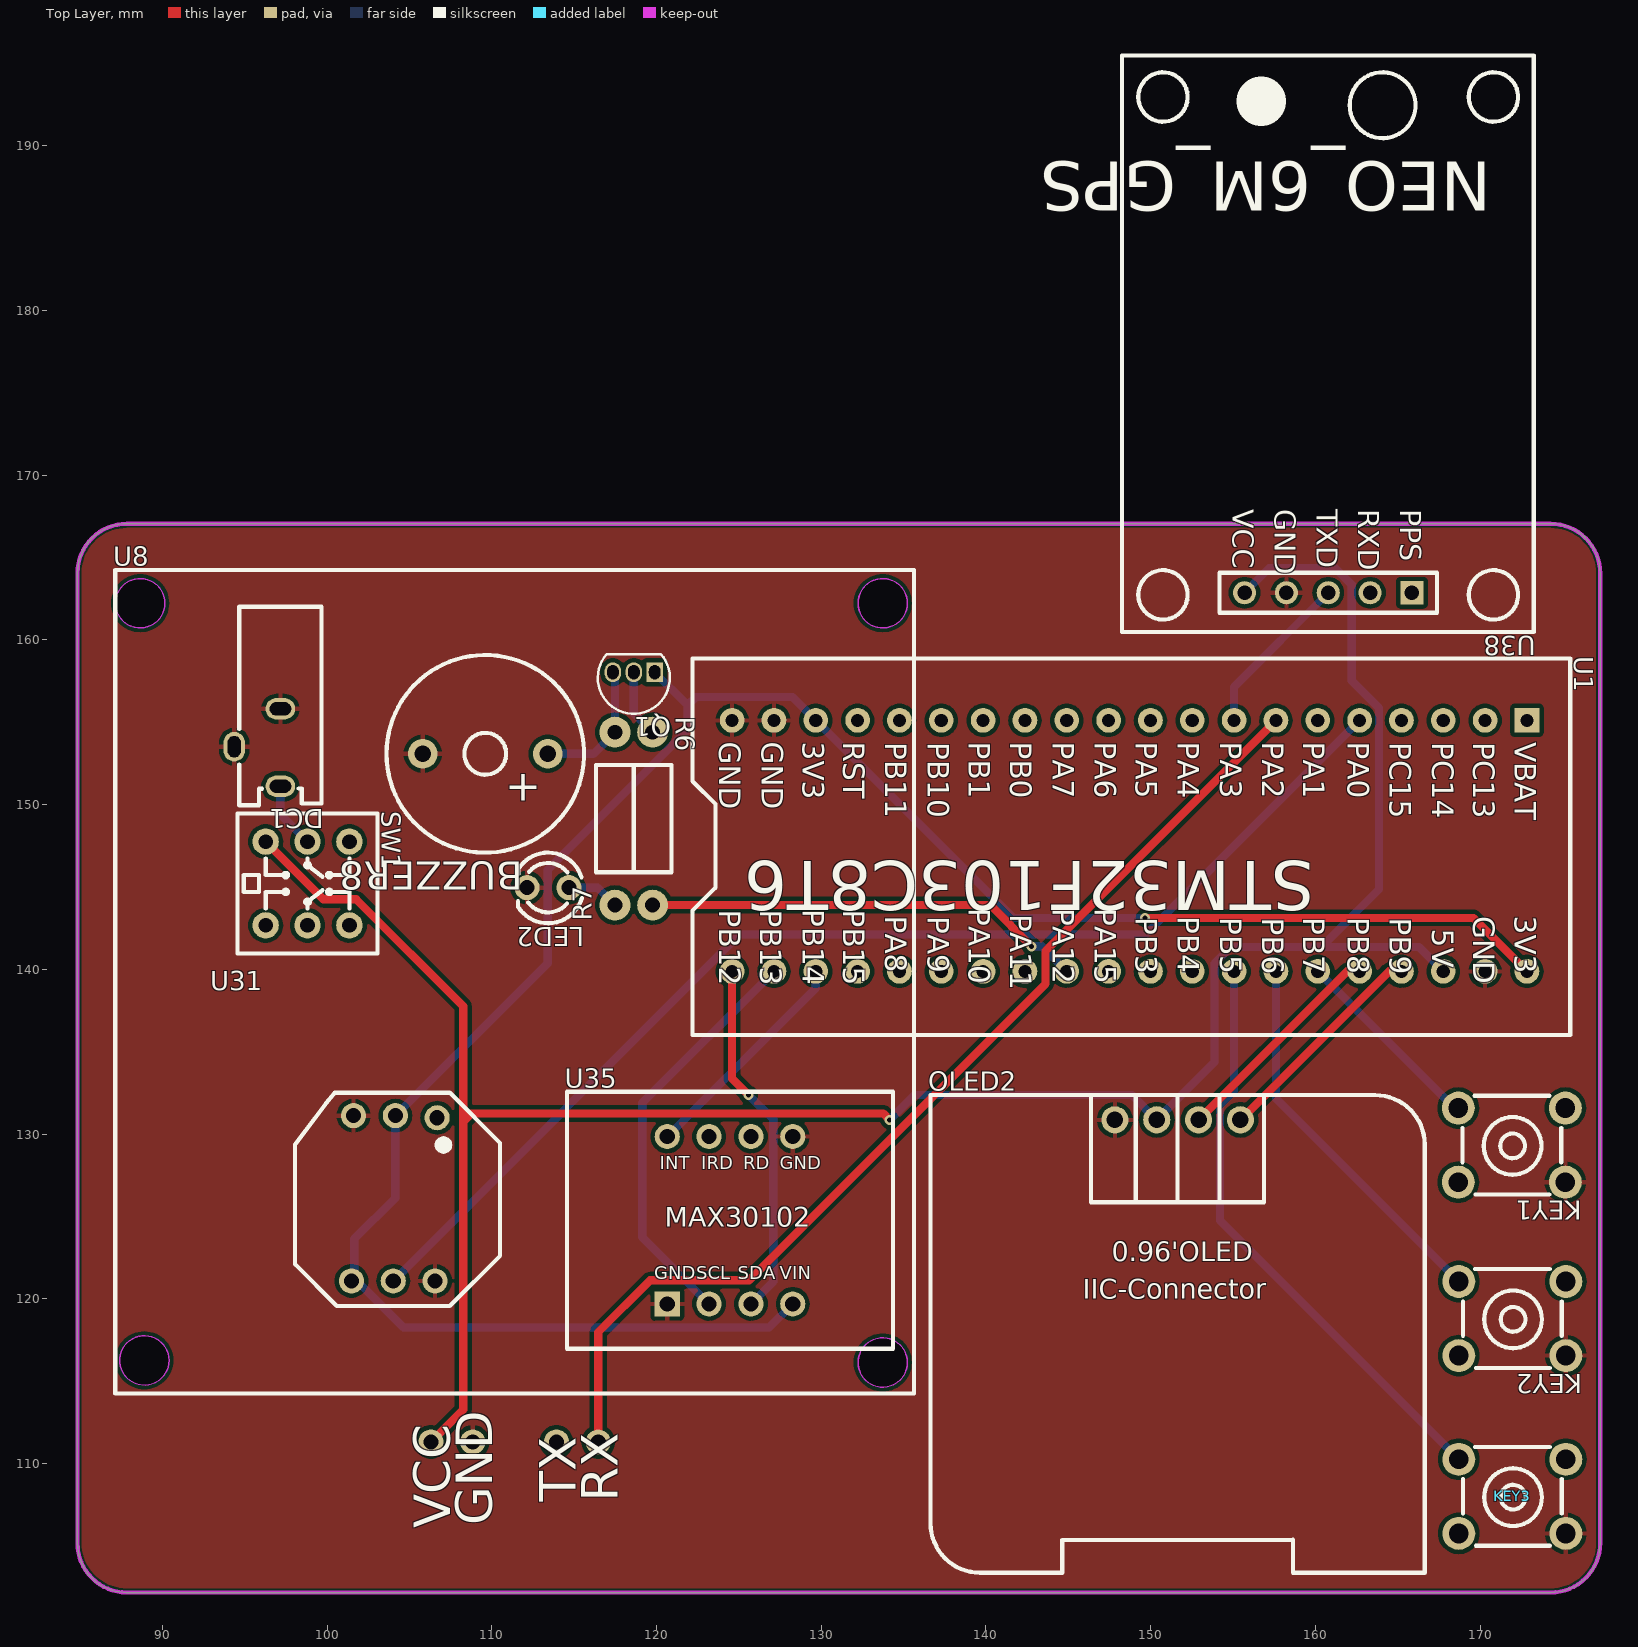
[diagram p0: Top Layer view]
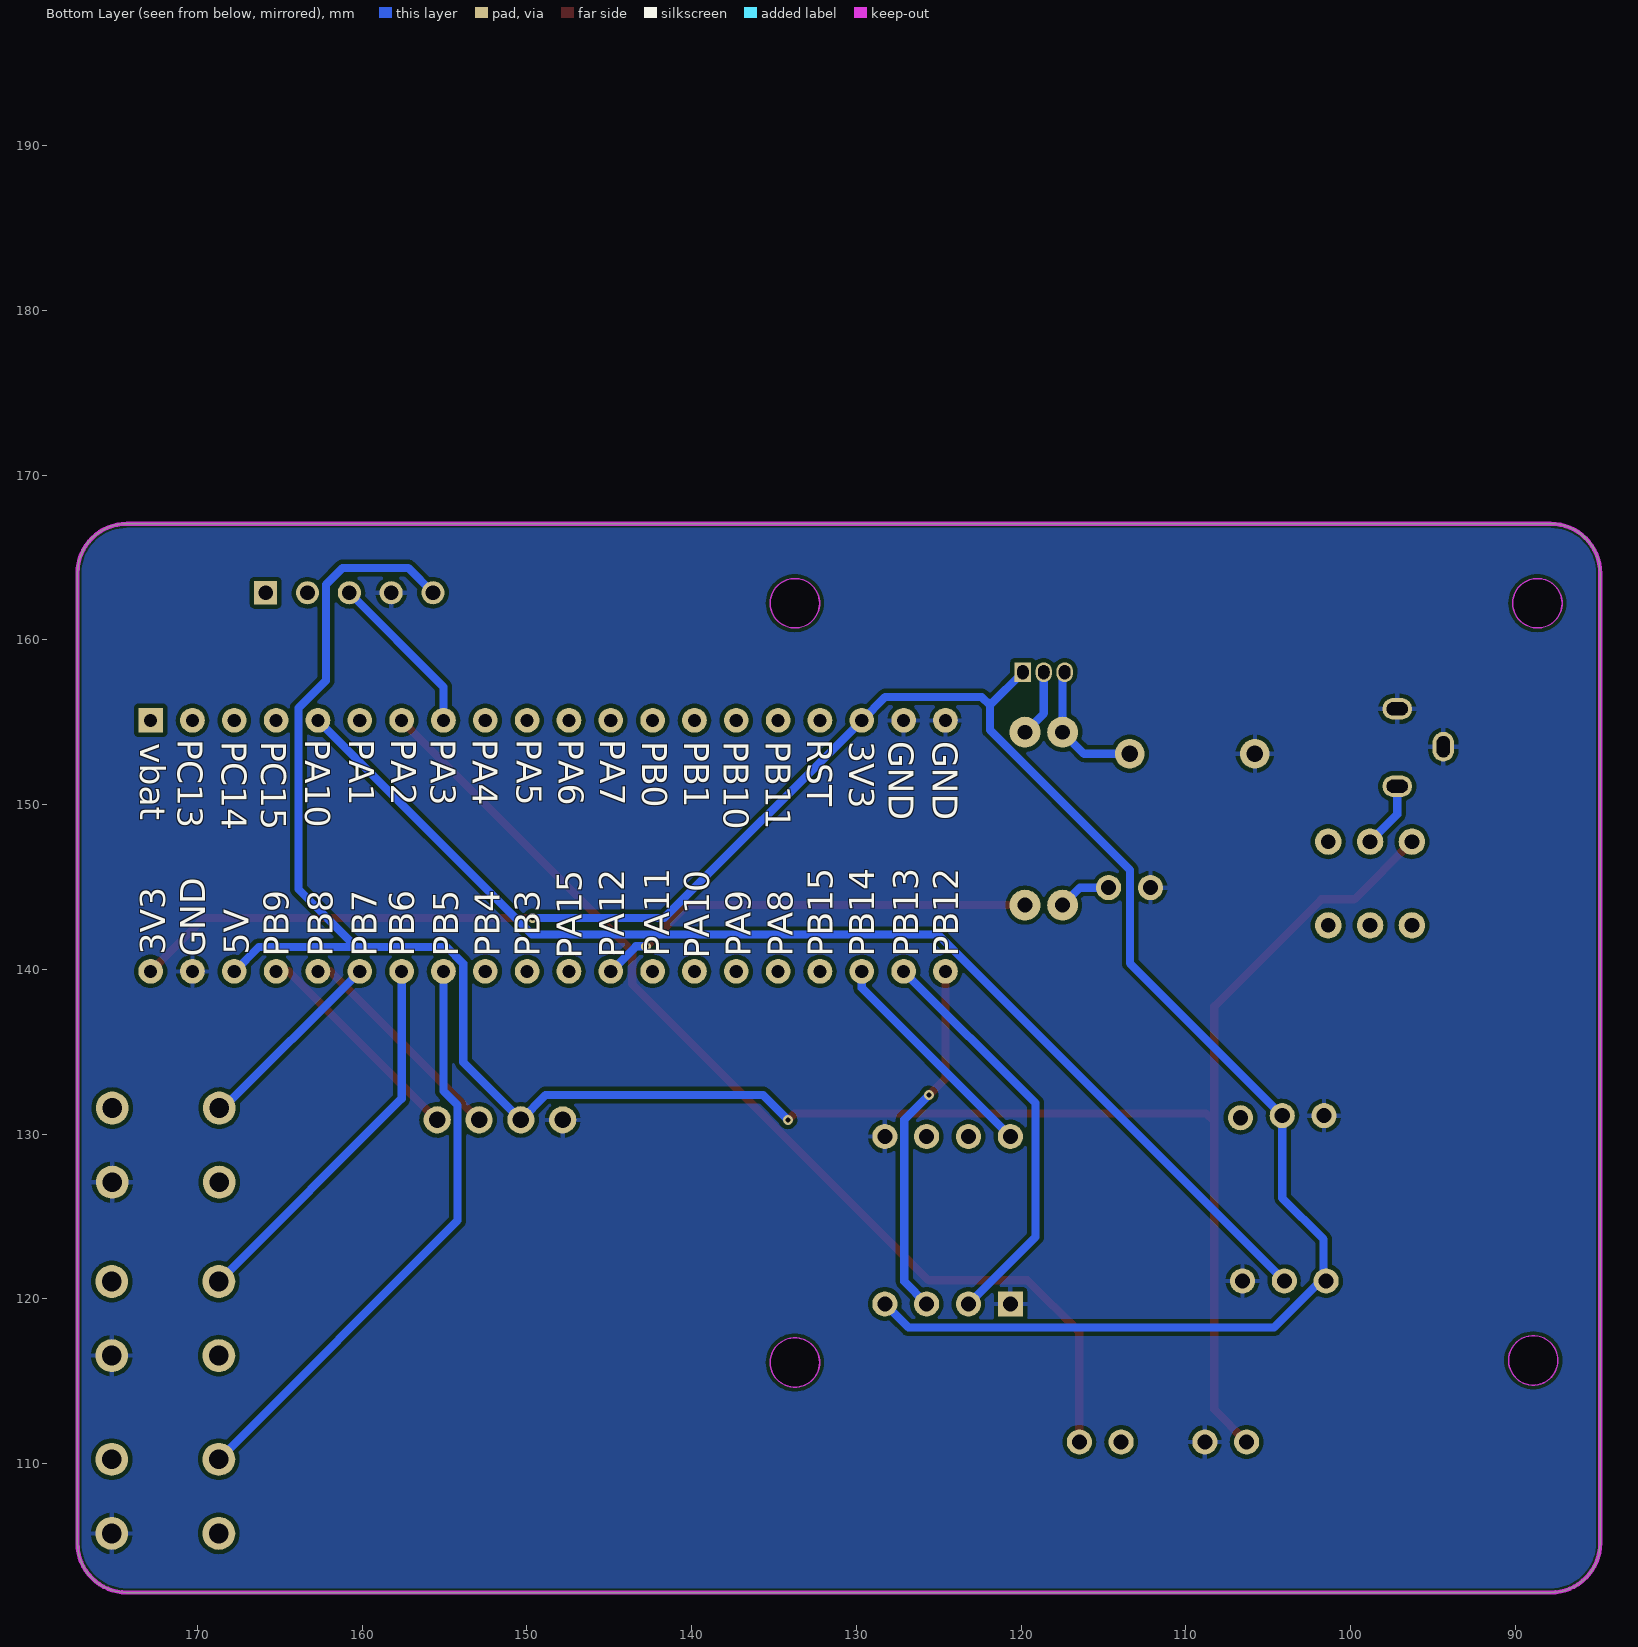
[diagram p1: Bottom Layer view, seen from below]
# Altium PCB MISC51078.pcbdoc
Units mm, origin at the board's own origin, x right, y up, seen from the top; angles counter-clockwise.
Board outline 92.46 x 64.9 mm, 2 copper layers (Top Layer, Bottom Layer), stack 1.58 mm thick; 16 components, 20 nets, 99 pads, 10 vias.

## Layer stack, top to bottom
Top Solder Mask Layer: solder mask 0.01, Dk 3.3
Top Layer: signal copper 0.035
Dielectric1: surface 1.51, FR4, Dk 4.5
Bottom Layer: signal copper 0.035
Bottom Solder Mask Layer: solder mask 0.01, Dk 3.3

## Board outline
87.836,167.056 ccw(c87.836,164.056) 84.836,164.056 84.836,105.159 ccw(c87.836,105.159) 87.836,102.159 174.292,102.159 ccw(c174.292,105.159) 177.292,105.159 177.292,164.056 ccw(c174.292,164.056) 174.292,167.056 87.836,167.056

## Design rules (kind name [scope] priority, off if disabled: settings)
BoardOutlineClearance copperThickness2oz_1 [All] p2 off: genericclearance=0.203 ignorepadtopadclearanceinfootprint=FALSE except(0: Arc-SplitContinuation Track-SplitContinuation SMDPad-SplitContinuation THPad-SplitContinuation Via-SplitContinuation Fill-SplitContinuation Region-SplitContinuation Poly-SplitContinuation Text-SplitContinuation Hole-SplitContinuation; 0.152: Arc-CutoutEdge Track-CutoutEdge SMDPad-CutoutEdge THPad-CutoutEdge Via-CutoutEdge Text-CutoutEdge; 0.175: Hole-OutlineEdge Hole-CutoutEdge; 0.254: Poly-OutlineEdge Poly-CutoutEdge; 0.3: Arc-OutlineEdge Track-OutlineEdge SMDPad-OutlineEdge THPad-OutlineEdge Via-OutlineEdge Fill-OutlineEdge Region-OutlineEdge Text-OutlineEdge Fill-CutoutEdge Region-CutoutEdge)
BoardOutlineClearance Plane_innerPlane_1 [All] p4 off: genericclearance=0.102 ignorepadtopadclearanceinfootprint=FALSE except(0: Arc-SplitContinuation Track-SplitContinuation SMDPad-SplitContinuation THPad-SplitContinuation Via-SplitContinuation Fill-SplitContinuation Region-SplitContinuation Poly-SplitContinuation Text-SplitContinuation Hole-SplitContinuation; 0.152: Arc-CutoutEdge Track-CutoutEdge SMDPad-CutoutEdge THPad-CutoutEdge Via-CutoutEdge Text-CutoutEdge; 0.175: Hole-OutlineEdge Hole-CutoutEdge; 0.254: Poly-OutlineEdge Poly-CutoutEdge; 0.3: Arc-OutlineEdge Track-OutlineEdge SMDPad-OutlineEdge THPad-OutlineEdge Via-OutlineEdge Fill-OutlineEdge Region-OutlineEdge Text-OutlineEdge Fill-CutoutEdge Region-CutoutEdge)
BoardOutlineClearance Copper_copperRegion_1 [All] p6 off: genericclearance=0.102 ignorepadtopadclearanceinfootprint=FALSE except(0: Arc-SplitContinuation Track-SplitContinuation SMDPad-SplitContinuation THPad-SplitContinuation Via-SplitContinuation Fill-SplitContinuation Region-SplitContinuation Poly-SplitContinuation Text-SplitContinuation Hole-SplitContinuation; 0.152: Arc-CutoutEdge Track-CutoutEdge SMDPad-CutoutEdge THPad-CutoutEdge Via-CutoutEdge Text-CutoutEdge; 0.175: Hole-OutlineEdge Hole-CutoutEdge; 0.254: Poly-OutlineEdge Poly-CutoutEdge; 0.3: Arc-OutlineEdge Track-OutlineEdge SMDPad-OutlineEdge THPad-OutlineEdge Via-OutlineEdge Fill-OutlineEdge Region-OutlineEdge Text-OutlineEdge Fill-CutoutEdge Region-CutoutEdge)
BoardOutlineClearance copperThickness1oz_1 [All] p8: genericclearance=0.102 ignorepadtopadclearanceinfootprint=FALSE except(0: Arc-SplitContinuation Track-SplitContinuation SMDPad-SplitContinuation THPad-SplitContinuation Via-SplitContinuation Fill-SplitContinuation Region-SplitContinuation Poly-SplitContinuation Text-SplitContinuation Hole-SplitContinuation; 0.152: Arc-CutoutEdge Track-CutoutEdge SMDPad-CutoutEdge THPad-CutoutEdge Via-CutoutEdge Text-CutoutEdge; 0.175: Hole-OutlineEdge Hole-CutoutEdge; 0.254: Poly-OutlineEdge Poly-CutoutEdge; 0.3: Arc-OutlineEdge Track-OutlineEdge SMDPad-OutlineEdge THPad-OutlineEdge Via-OutlineEdge Fill-OutlineEdge Region-OutlineEdge Text-OutlineEdge Fill-CutoutEdge Region-CutoutEdge)
Clearance copperThickness2oz [All] p1 off: gap=0.203 ignorepadtopadclearanceinfootprint=FALSE except(0.152: SMDPad-Track SMDPad-SMDPad THPad-Track SMDPad-THPad THPad-THPad Track-Via SMDPad-Via THPad-Via Via-Via Fill-SMDPad Region-SMDPad Fill-THPad Region-THPad Fill-Via Region-Via Fill-Fill Fill-Region Region-Region Arc-Track Arc-SMDPad Arc-THPad Arc-Via Fill-Arc Region-Arc Arc-Arc Text-Track SMDPad-Text Text-THPad Text-Via Fill-Text Region-Text Arc-Text Text-Text; 0.175: Hole-Track Hole-SMDPad Hole-THPad Hole-Via Fill-Hole Region-Hole Hole-Arc Hole-Text; 0.254: Poly-Track Poly-SMDPad Poly-THPad Poly-Via Poly-Fill Poly-Region Poly-Poly Poly-Arc Poly-Text Poly-Hole; 0.3: Fill-Track Region-Track)
Clearance Plane_innerPlane [All] p3 off: gap=0.102 ignorepadtopadclearanceinfootprint=FALSE except(0.152: SMDPad-Track SMDPad-SMDPad THPad-Track SMDPad-THPad THPad-THPad Track-Via SMDPad-Via THPad-Via Via-Via Fill-SMDPad Region-SMDPad Fill-THPad Region-THPad Fill-Via Region-Via Fill-Fill Fill-Region Region-Region Arc-Track Arc-SMDPad Arc-THPad Arc-Via Fill-Arc Region-Arc Arc-Arc Text-Track SMDPad-Text Text-THPad Text-Via Fill-Text Region-Text Arc-Text Text-Text; 0.175: Hole-Track Hole-SMDPad Hole-THPad Hole-Via Fill-Hole Region-Hole Hole-Arc Hole-Text; 0.254: Poly-Track Poly-SMDPad Poly-THPad Poly-Via Poly-Fill Poly-Region Poly-Poly Poly-Arc Poly-Text Poly-Hole; 0.3: Fill-Track Region-Track)
Clearance Copper_copperRegion [All] p5 off: gap=0.102 ignorepadtopadclearanceinfootprint=FALSE except(0.152: SMDPad-Track SMDPad-SMDPad THPad-Track SMDPad-THPad THPad-THPad Track-Via SMDPad-Via THPad-Via Via-Via Fill-SMDPad Region-SMDPad Fill-THPad Region-THPad Fill-Via Region-Via Fill-Fill Fill-Region Region-Region Arc-Track Arc-SMDPad Arc-THPad Arc-Via Fill-Arc Region-Arc Arc-Arc Text-Track SMDPad-Text Text-THPad Text-Via Fill-Text Region-Text Arc-Text Text-Text; 0.175: Hole-Track Hole-SMDPad Hole-THPad Hole-Via Fill-Hole Region-Hole Hole-Arc Hole-Text; 0.254: Poly-Track Poly-SMDPad Poly-THPad Poly-Via Poly-Fill Poly-Region Poly-Poly Poly-Arc Poly-Text Poly-Hole; 0.3: Fill-Track Region-Track)
Clearance copperThickness1oz [All] p7: gap=0.102 ignorepadtopadclearanceinfootprint=FALSE except(0.152: SMDPad-Track SMDPad-SMDPad THPad-Track SMDPad-THPad THPad-THPad Track-Via SMDPad-Via THPad-Via Via-Via Fill-SMDPad Region-SMDPad Fill-THPad Region-THPad Fill-Via Region-Via Fill-Fill Fill-Region Region-Region Arc-Track Arc-SMDPad Arc-THPad Arc-Via Fill-Arc Region-Arc Arc-Arc Text-Track SMDPad-Text Text-THPad Text-Via Fill-Text Region-Text Arc-Text Text-Text; 0.175: Hole-Track Hole-SMDPad Hole-THPad Hole-Via Fill-Hole Region-Hole Hole-Arc Hole-Text; 0.254: Poly-Track Poly-SMDPad Poly-THPad Poly-Via Poly-Fill Poly-Region Poly-Poly Poly-Arc Poly-Text Poly-Hole; 0.3: Fill-Track Region-Track)
DiffPairsRouting differentialPair [All] p1: maxlimit=0.152 minlimit=0.152 mostfreqgap=0.152 toplayer_minwidth=0.127 toplayer_prefwidth=0.254 toplayer_maxwidth=2.54 toplayer_mingap=0.152 toplayer_prefgap=0.152 toplayer_maxgap=0.152 bottomlayer_minwidth=0.127 bottomlayer_prefwidth=0.254 bottomlayer_maxwidth=2.54 bottomlayer_mingap=0.152 bottomlayer_prefgap=0.152 bottomlayer_maxgap=0.152 maxuncoupledlength=0.254
HoleToHoleClearance otherClearance [All] p1: gap=0.3 allowstackedmicrovias=TRUE
Length netLength [All] p1: minlimit=0 maxlimit=0
PasteMaskExpansion pasteMaskExpansion [All] p1: expansion=0
PlaneConnect innerPlane [All] p1: planeconnectstyle=Relief reliefexpansion=0.508 reliefentries=4 reliefconductorwidth=0.254 reliefairgap=0.254
PolygonConnect copperRegion [All] p1: connectstyle=Relief reliefconductorwidth=0.254 reliefentries=4 polygonreliefangle="90 Angle" airgapwidth=0.254 via.connectstyle=Relief via.reliefconductorwidth=0.254 via.reliefentries=4 via.polygonreliefangle="90 Angle" via.airgapwidth=0.254
RoutingVias viaSize [All] p1: holewidth=0.305 width=0.61 viastyle="Through Hole" minholewidth=0.3 minwidth=0.5 maxholewidth=6.3 maxwidth=10
SolderMaskExpansion solderMaskExpansion [IsVia] p1: expansion=-25.4 istentingtop=TRUE
SolderMaskExpansion solderMaskExpansion [All] p2: expansion=0.051 istentingtop=FALSE
Width copperThickness2oz_2 [All] p1 off: maxlimit=2.54 minlimit=0.203 preferedwidth=0.254
Width copperThickness1oz_2 [All] p2: maxlimit=2.54 minlimit=0.127 preferedwidth=0.5

## Components (designator, comment, footprint, x,y, rotation, side; value= is the part's Value field where it differs from the comment)
BUZZER8 "buzzer-12X9" BUZ-TH_BD12.0-P7.60-D0.6-FD 109.601,153.086 r180 top
DC1 "DC002-1.3" DC-IN-TH_DC002-1.3 95.758,153.467 r180 top
KEY1 "按键开关6*6*8" KEY-TH_4P-L6.0-W6.0-P4.50-LS7.5 171.929,129.328 r180 top
KEY2 "按键开关6*6*8" KEY-TH_4P-L6.0-W6.0-P4.50-LS7.5 171.958,118.796 r180 top
KEY3 "按键开关6*6*8" KEY-TH_4P-L6.0-W6.0-P4.50-LS7.5 171.958,108.001 r180 top
LED2 "" LED_TH-3mm 113.411,144.958 r180 top
OLED2 "0.96OLED_4P_MODULE_JX" 0.96OLED_4P 151.638,130.861 r0 top
Q1 "S8550" TO-92-3_L4.5-W3.5-P1.27-L 118.618,158.039 r180 top
R6 "" RES-TH_BD2.3-L6.5-P10.50-D0.5 119.761,149.149 r270 top
R7 "" RES-TH_BD2.3-L6.5-P10.50-D0.5 117.475,149.149 r90 top
SW1 "" 自锁开关8.5*8.5 101.346,147.752 r270 top
U1 "STM32F103C8T6-Bluepill" STM32F103C8T6-BLUEPILL 147.447,147.498 r270 top
U8 "SIM900A" SIM900A 111.379,139.243 r0 top
U31 "" "AGR12 表面压力传感器" 101.854,124.892 r0 top
U35 "" MAX30102 120.65,129.845 r0 top
U38 "" NEO_6M_GPS模块 160.909,179.375 r180 top

## Footprints (in the part's own frame and the unit in brackets; to place one, negate y for a bottom-side part, rotate by r counter-clockwise, add the part's x,y. Pads: shape width x height; smd on the part's side, far side on the other; paste and mask are expansions set on the pad)
0.96OLED_4P [mm]
  round 1.65 hole 1 copper offset 0,0 paste+0 mask+0.051: 1(-3.81,-0.001) 2(-1.27,0.002) 3(1.27,0.002) 4(3.81,0.002)
  silkscreen extent -15,-27.5 15,1.5
"AGR12 表面压力传感器" [mil]
  round 60 hole 36: 1(190,240) 2(90,245) 3(-10,245) 4(-15,-150) 5(85,-150) 6(185,-150)
  silkscreen extent -150,-210 340,300
BUZ-TH_BD12.0-P7.60-D0.6-FD [mm]
  round 1.801 hole 1.001 paste+0 mask+0.051: 1(-3.8,0) 2(3.8,0)
  silkscreen extent -6,-6 6,6
DC-IN-TH_DC002-1.3 [mm]
  oval 1.8x1.3 hole 0.8 slot 1.3 at 0 deg paste+0 mask+0.05: 1(-1.4,2.35) 3(-1.4,-2.35)
  oval 1.3x1.8 hole 0.8 slot 1.3 at 90 deg paste+0 mask+0.05: 2(1.4,-0.05)
  silkscreen extent -3.9,-8.55 1.1,3.5
KEY-TH_4P-L6.0-W6.0-P4.50-LS7.5 [mm]
  round 2 hole 1.2 paste+0 mask+0.051: 1(-3.25,-2.25) 2(3.25,-2.25) 3(3.25,2.25) 4(-3.25,2.25)
  silkscreen extent -3,-3 3,3
LED_TH-3mm [mil]
  round 60 hole 36 paste+0 mask+2: 1(-50,0) 2(50,0)
  silkscreen extent -81,-84 72,85
MAX30102 [mil]
  round 60 hole 36 paste+0 mask+4: 1(300.01,-400.01) 2(200.01,-400.01) 3(100.01,-400.01) 5(0.01,-0.01) 6(100.01,-0.01) 7(200.01,-0.01) 8(300.01,-0.01)
  rect 60x60 hole 36 paste+0 mask+4: 4(0.01,-400.01)
  silkscreen extent -240,-507 540,107
NEO_6M_GPS模块 [mil]
  rect 55.1x55.1 hole 35 paste+0 mask+2: 1(-195,650)
  round 55.1 hole 35 paste+0 mask+2: 2(-95,650) 3(5,650) 4(105,650) 5(205,650)
  silkscreen extent -486,-634 498,744
RES-TH_BD2.3-L6.5-P10.50-D0.5 [mil]
  round 74 hole 35.4 paste+0 mask+2: 1(-206.69,0) 2(206.69,0)
  silkscreen extent -128,-45 128,45
SIM900A [mil]
  round 60 hole 36 paste+0 mask+2: 1(-200,-1100) 2(-100,-1100) 3(100,-1100) 4(200,-1100)
  Board Outline Layer circle w0.1: c-895,905 r59.05
  Board Outline Layer circle w0.1: c880,905 r59.05
  Board Outline Layer circle w0.1: c-885,-905 r59.05
  Board Outline Layer circle w0.1: c880,-910 r59.05
  Board Outline Layer region: -835.95,905 -841.79,879.38 -858.18,858.83 -881.86,847.43 -908.14,847.43 -931.82,858.83 -948.21,879.38 -954.05,905 -954.05,905 -948.21,930.62 -931.82,951.17 -908.14,962.57 -881.86,962.57 -858.18,951.17 -841.79,930.62 -835.95,905
  Board Outline Layer region: -835.95,905 -836.34,898.14 -837.54,891.38 -839.51,884.8 -842.23,878.5 -845.66,872.55 -849.76,867.04 -854.47,862.04 -859.73,857.63 -865.47,853.86 -871.61,850.77 -878.06,848.43 -884.75,846.84 -891.57,846.04 -898.43,846.04 -905.25,846.84 -911.94,848.43 -918.39,850.77 -924.53,853.86 -930.27,857.63 -935.53,862.04 -940.24,867.04 -944.34,872.55 -947.77,878.5 -950.49,884.8 -952.46,891.38 -953.66,898.14 -954.05,905 -953.66,911.86 -952.46,918.62 -950.49,925.2 -947.77,931.5 -944.34,937.45 -940.24,942.96 -935.53,947.96 -930.27,952.37 -924.53,956.14 -918.39,959.23 -911.94,961.57 -905.25,963.16 -898.43,963.96 -891.57,963.96 -884.75,963.16 -878.06,961.57 -871.61,959.23 -865.47,956.14 -859.73,952.37 -854.47,947.96 -849.76,942.96 -845.66,937.45 -842.23,931.5 -839.51,925.2 -837.54,918.62 -836.34,911.86
  Board Outline Layer region: 939.06,905 933.21,879.38 916.82,858.83 893.14,847.43 866.86,847.43 843.18,858.83 826.79,879.38 820.94,905 820.94,905 826.79,930.62 843.18,951.17 866.86,962.57 893.14,962.57 916.82,951.17 933.21,930.62 939.06,905
  Board Outline Layer region: 939.06,905 938.66,898.14 937.46,891.38 935.49,884.8 932.77,878.5 929.34,872.55 925.24,867.04 920.53,862.04 915.27,857.63 909.53,853.86 903.39,850.77 896.94,848.43 890.25,846.84 883.43,846.04 876.57,846.04 869.75,846.84 863.06,848.43 856.61,850.77 850.47,853.86 844.73,857.63 839.47,862.04 834.76,867.04 830.66,872.55 827.23,878.5 824.51,884.8 822.54,891.38 821.34,898.14 820.94,905 821.34,911.86 822.54,918.62 824.51,925.2 827.23,931.5 830.66,937.45 834.76,942.96 839.47,947.96 844.73,952.37 850.47,956.14 856.61,959.23 863.06,961.57 869.75,963.16 876.57,963.96 883.43,963.96 890.25,963.16 896.94,961.57 903.39,959.23 909.53,956.14 915.27,952.37 920.53,947.96 925.24,942.96 929.34,937.45 932.77,931.5 935.49,925.2 937.46,918.62 938.66,911.86
  Board Outline Layer region: -825.95,-905 -831.79,-930.62 -848.18,-951.17 -871.86,-962.57 -898.14,-962.57 -921.82,-951.17 -938.21,-930.62 -944.05,-905 -944.05,-905 -938.21,-879.38 -921.82,-858.83 -898.14,-847.43 -871.86,-847.43 -848.18,-858.83 -831.79,-879.38 -825.95,-905
  Board Outline Layer region: -825.95,-905 -826.34,-911.86 -827.54,-918.62 -829.51,-925.2 -832.23,-931.5 -835.66,-937.45 -839.76,-942.96 -844.47,-947.96 -849.73,-952.37 -855.47,-956.14 -861.61,-959.23 -868.06,-961.57 -874.75,-963.16 -881.57,-963.96 -888.43,-963.96 -895.25,-963.16 -901.94,-961.57 -908.39,-959.23 -914.53,-956.14 -920.27,-952.37 -925.53,-947.96 -930.24,-942.96 -934.34,-937.45 -937.77,-931.5 -940.49,-925.2 -942.46,-918.62 -943.66,-911.86 -944.05,-905 -943.66,-898.14 -942.46,-891.38 -940.49,-884.8 -937.77,-878.5 -934.34,-872.55 -930.24,-867.04 -925.53,-862.04 -920.27,-857.63 -914.53,-853.86 -908.39,-850.77 -901.94,-848.43 -895.25,-846.84 -888.43,-846.04 -881.57,-846.04 -874.75,-846.84 -868.06,-848.43 -861.61,-850.77 -855.47,-853.86 -849.73,-857.63 -844.47,-862.04 -839.76,-867.04 -835.66,-872.55 -832.23,-878.5 -829.51,-884.8 -827.54,-891.38 -826.34,-898.14
  Board Outline Layer region: 939.06,-910 933.21,-935.62 916.82,-956.17 893.14,-967.57 866.86,-967.57 843.18,-956.17 826.79,-935.62 820.94,-910 820.94,-910 826.79,-884.38 843.18,-863.83 866.86,-852.43 893.14,-852.43 916.82,-863.83 933.21,-884.38 939.06,-910
  Board Outline Layer region: 939.06,-910 938.66,-916.86 937.46,-923.62 935.49,-930.2 932.77,-936.5 929.34,-942.45 925.24,-947.96 920.53,-952.96 915.27,-957.37 909.53,-961.14 903.39,-964.23 896.94,-966.57 890.25,-968.16 883.43,-968.96 876.57,-968.96 869.75,-968.16 863.06,-966.57 856.61,-964.23 850.47,-961.14 844.73,-957.37 839.47,-952.96 834.76,-947.96 830.66,-942.45 827.23,-936.5 824.51,-930.2 822.54,-923.62 821.34,-916.86 820.94,-910 821.34,-903.14 822.54,-896.38 824.51,-889.8 827.23,-883.5 830.66,-877.55 834.76,-872.04 839.47,-867.04 844.73,-862.63 850.47,-858.86 856.61,-855.77 863.06,-853.43 869.75,-851.84 876.57,-851.04 883.43,-851.04 890.25,-851.84 896.94,-853.43 903.39,-855.77 909.53,-858.86 915.27,-862.63 920.53,-867.04 925.24,-872.04 929.34,-877.55 932.77,-883.5 935.49,-889.8 937.46,-896.38 938.66,-903.14
  Multi-Layer board cut-out: -835.95,905 -841.79,879.38 -858.18,858.83 -881.86,847.43 -908.14,847.43 -931.82,858.83 -948.21,879.38 -954.05,905 -954.05,905 -948.21,930.62 -931.82,951.17 -908.14,962.57 -881.86,962.57 -858.18,951.17 -841.79,930.62 -835.95,905
  Multi-Layer board cut-out: 939.06,905 933.21,879.38 916.82,858.83 893.14,847.43 866.86,847.43 843.18,858.83 826.79,879.38 820.94,905 820.94,905 826.79,930.62 843.18,951.17 866.86,962.57 893.14,962.57 916.82,951.17 933.21,930.62 939.06,905
  Multi-Layer board cut-out: -825.95,-905 -831.79,-930.62 -848.18,-951.17 -871.86,-962.57 -898.14,-962.57 -921.82,-951.17 -938.21,-930.62 -944.05,-905 -944.05,-905 -938.21,-879.38 -921.82,-858.83 -898.14,-847.43 -871.86,-847.43 -848.18,-858.83 -831.79,-879.38 -825.95,-905
  Multi-Layer board cut-out: 939.06,-910 933.21,-935.62 916.82,-956.17 893.14,-967.57 866.86,-967.57 843.18,-956.17 826.79,-935.62 820.94,-910 820.94,-910 826.79,-884.38 843.18,-863.83 866.86,-852.43 893.14,-852.43 916.82,-863.83 933.21,-884.38 939.06,-910
  silkscreen extent -955,-984 955,984
STM32F103C8T6-BLUEPILL [mm]
  rect 1.5x1.5 hole 0.8 paste+0 mask+0.051: 1(-7.62,25.4)
  round 1.5 hole 0.8 paste+0 mask+0.051: 2(-7.62,22.86) 3(-7.62,20.32) 4(-7.62,17.78) 5(-7.62,15.24) 6(-7.62,12.7) 7(-7.62,10.16) 8(-7.62,7.62) 9(-7.62,5.08) 10(-7.62,2.54) 11(-7.62,0) 12(-7.62,-2.54) 13(-7.62,-5.08) 14(-7.62,-7.62) 15(-7.62,-10.16) 16(-7.62,-12.7) 17(-7.62,-15.24) 18(-7.62,-17.78) 19(-7.62,-20.32) 20(-7.62,-22.86) 21(7.62,-22.86) 22(7.62,-20.32) 23(7.62,-17.78) 24(7.62,-15.24) 25(7.62,-12.7) 26(7.62,-10.16) 27(7.62,-7.62) 28(7.62,-5.08) 29(7.62,-2.54) 30(7.62,0) 31(7.62,2.54) 32(7.62,5.08) 33(7.62,7.62) 34(7.62,10.16) 35(7.62,12.7) 36(7.62,15.24) 37(7.62,17.78) 38(7.62,20.32) 39(7.62,22.86) 40(7.62,25.4)
  silkscreen extent -11.38,-25.26 11.48,28.03
TO-92-3_L4.5-W3.5-P1.27-L [mm]
  rect 1x1.2 hole 0.7 slot 0.85 at 90 deg paste+0 mask+0.051: 1(-1.27,0)
  oval 1x1.2 hole 0.7 slot 0.85 at 90 deg paste+0 mask+0.051: 2(0,0) 3(1.27,0)
  silkscreen extent -2.19,-1.1 2.19,2.52
自锁开关8.5*8.5 [mm]
  round 1.6 hole 0.9: 1(0,0) 2(0,-2.54) 3(0,-5.08) 4(5.08,-5.08) 5(5.08,-2.54) 6(5.08,0)
  silkscreen extent -1.71,-6.79 6.79,1.71

## Via types
v1: diameter 0.61, hole 0.305, Top Layer to Bottom Layer, 10 vias

## Nets (pads, with @x,y where several pads share a name; then routed paths per layer and width w, separated by ;. In a path a pad name is that pad's centre, name@x,y a point inside that pad or via, vN(x,y) a via of type N, cw(c..) or ccw(c..) an arc to the next point about the centre after c; other vN are vias at no path point)
$1N783: DC1.1 SW1.2 | length 4
  Bottom Layer w0.5: DC1.1 97.158,149.4 SW1.2
$1N823: BUZZER8.1 Q1.3 R7.2 | length 8.3
  Bottom Layer w0.5: BUZZER8.1 116.162,153.086 R7.2 117.475,157.912 Q1.3
$1N824: LED2.1 R7.1 | length 3.2
  Bottom Layer w0.5: LED2.1 116.416,144.958 R7.1
$1N825: Q1.2 R6.1 | length 4.1
  Bottom Layer w0.5: Q1.2 118.618,155.542 R6.1
+5V: OLED2.2 SW1.3 U1.38 U8.1 U38.5 | length 144.7
  Top Layer w0.5: SW1.3 99.766,144.252 101.766,144.252 108.266,137.752 108.266,130.752 ; U8.1 108.266,113.27 108.266,130.752 ; v1(134.156,130.862) 133.766,131.252 108.766,131.252 108.266,130.752
  Bottom Layer w0.5: v1(134.156,130.862) 135.656,132.362 148.868,132.362 OLED2.2 153.868,134.362 153.868,140.362 154.868,141.362 160.368,141.362 ; U38.5 157.199,164.362 161.205,164.362 162.205,163.362 162.205,157.525 163.868,155.862 163.868,144.862 160.368,141.362 ; U1.38 166.283,141.362 160.368,141.362
BEEP: R6.2 U1.29 | length 26.8
  Top Layer w0.5: R6.2 140.261,143.899 v1(142.761,141.399)
  Bottom Layer w0.5: v1(142.761,141.399) 143.386,141.399 U1.29
GND: BUZZER8.2 DC1.2 DC1.3 KEY1.4 KEY2.4 KEY3.4 LED2.2 OLED2.1 U1.19 U1.20 U1.39 U8.2 U31.3 U31.6 U35.4 U35.8 U38.4
  other v1: 106.553,121.082 101.473,131.115
KEY1: KEY3.2 U1.33 | length 36
  Bottom Layer w0.5: U1.33 155.067,132.61 154.208,131.751 154.208,124.751 KEY3.2
KEY2: KEY2.2 U1.34 | length 23.4
  Bottom Layer w0.5: U1.34 157.607,132.147 KEY2.2
KEY3: KEY1.2 U1.35 | length 12
  Bottom Layer w0.5: U1.35 168.447,131.578 KEY1.2
PA3: U1.8 U38.3 | length 10.1
  Bottom Layer w0.5: U1.8 155.067,157.15 U38.3
PB8: OLED2.3 U1.36 | length 13.5
  Top Layer w0.5: OLED2.3 161.924,139.878 U1.36
PB9: OLED2.4 U1.37 | length 13.5
  Top Layer w0.5: OLED2.4 164.464,139.878 U1.37
PB12: U1.21 U35.2 | length 21.8
  Top Layer w0.5: U1.21 124.587,133.378 v1(125.587,132.378)
  Bottom Layer w0.5: v1(125.587,132.378) 127.087,130.878 127.087,121.042 U35.2
PB13: U1.22 U35.3 | length 25.2
  Bottom Layer w0.5: U35.3 119.127,123.748 119.127,131.878 U1.22
PB14: U1.23 U35.5 | length 13.8
  Bottom Layer w0.5: U35.5 129.667,138.862 U1.23
PRESS: U1.5 U31.5 | length 72.8
  Bottom Layer w0.5: v1(104.013,121.082) 125.049,142.118 149.687,142.118 U1.5
SIM900A_RX: U1.7 U8.4 | length 64.4
  Top Layer w0.5: U8.4 116.459,117.97 119.607,121.118 125.607,121.118 143.607,139.118 143.607,141.118 U1.7
SIM900A_TX: U8.3
VCC: Q1.1 U1.18 U1.40 U31.2 U31.4 U35.1 | length 132.8
  Top Layer w0.5: v1(149.667,143.118) 169.607,143.118 U1.40
  Bottom Layer w0.5: v1(101.473,121.082) U31.4@101.64,121.249 ; Q1.1 121.888,156.039 ; U35.1 126.834,118.249 104.64,118.249 U31.4@101.64,121.249 ; v1(149.667,143.118) 141.667,143.118 U1.18 128.246,156.539 122.388,156.539 121.888,156.039 ; U31.4@101.64,121.249 101.64,123.615 104.14,126.115 U31.2 113.388,140.363 113.388,146.039 121.888,154.539 121.888,156.039
  other v1: 104.013,131.115
pads on no net: KEY1.1 KEY1.3 KEY2.1 KEY2.3 KEY3.1 KEY3.3 SW1.1 SW1.4 SW1.5 SW1.6 U1.1 U1.2 U1.3 U1.4 U1.6 U1.9 U1.10 U1.11 U1.12 U1.13 U1.14 U1.15 U1.16 U1.17 U1.24 U1.25 U1.26 U1.27 U1.28 U1.30 U1.31 U1.32 U31.1 U35.6 U35.7 U38.1 U38.2
copper on no net:
  other v1: 106.553,131.115

## Polygon pours and split planes (outlines as drawn)
GND on Top Layer (solid, remove dead copper, pour order 0): 80.391,172.009 80.391,95.428 197.612,95.428 197.612,172.009
GND on Bottom Layer (solid, remove dead copper, pour order 2): 76.2,172.009 76.2,97.333 186.817,97.333 186.817,172.009

## Keep-outs
Board Outline Layer:
  the board outline again, w0.254

## Silkscreen, mask and mechanical layers (free items; w line width, h text height)
Bottom Silkscreen Layer:
  text "RST" at 132.969,153.975 h1.52 r90
  text "PA7" at 145.542,153.975 h1.52 r90
  text "PA6" at 148.082,153.975 h1.52 r90
  text "PA5" at 150.622,153.975 h1.52 r90
  text "PA4" at 153.289,153.975 h1.52 r90
  text "PA3" at 155.829,153.975 h1.52 r90
  text "PA2" at 158.242,153.975 h1.52 r90
  text "PA1" at 160.782,153.975 h1.52 r90
  text "PA10" at 163.449,153.975 h1.52 r90
  text "PC13" at 171.196,153.975 h1.52 r90
  text "GND" at 125.349,153.848 h1.52 r90
  text "GND" at 128.016,153.848 h1.52 r90
  text "3V3" at 130.429,153.848 h1.52 r90
  text "PB11" at 135.509,153.848 h1.52 r90
  text "PB10" at 138.049,153.848 h1.52 r90
  text "PB1" at 140.462,153.848 h1.52 r90
  text "PB0" at 143.002,153.848 h1.52 r90
  text "PC15" at 166.116,153.848 h1.52 r90
  text "PC14" at 168.529,153.848 h1.52 r90
  text "vbat" at 173.482,153.721 h1.52 r90
  text "5V" at 166.878,140.894 h1.52 r270
  text "3V3" at 171.958,140.894 h1.52 r270
  text "PB12" at 123.825,140.767 h1.52 r270
  text "PB13" at 126.238,140.767 h1.52 r270
  text "PB14" at 128.905,140.767 h1.52 r270
  text "PB15" at 131.445,140.767 h1.52 r270
  text "PA8" at 133.858,140.767 h1.52 r270
  text "PA9" at 136.398,140.767 h1.52 r270
  text "PA11" at 141.351,140.767 h1.52 r270
  text "PB3" at 149.225,140.767 h1.52 r270
  text "PB4" at 151.638,140.767 h1.52 r270
  text "PB5" at 154.178,140.767 h1.52 r270
  text "PB6" at 156.845,140.767 h1.52 r270
  text "PB7" at 159.131,140.767 h1.52 r270
  text "PB8" at 161.798,140.767 h1.52 r270
  text "PB9" at 164.465,140.767 h1.52 r270
  text "GND" at 169.545,140.767 h1.52 r270
  text "PA12" at 144.094,140.691 h1.52 r270
  text "PA10" at 138.938,140.64 h1.52 r270
  text "PA15" at 146.685,140.64 h1.52 r270

## Dimensions
110.534,131.115 to 110.534,121.115 on Document Layer
95.504,119.558 to 95.504,132.558 on Document Layer
100.457,134.798 to 107.457,134.798 on Document Layer
82.169,176.2 to 182.169,176.2 on Document Layer
181.61,176.2 to 181.61,76.2 on Document Layer